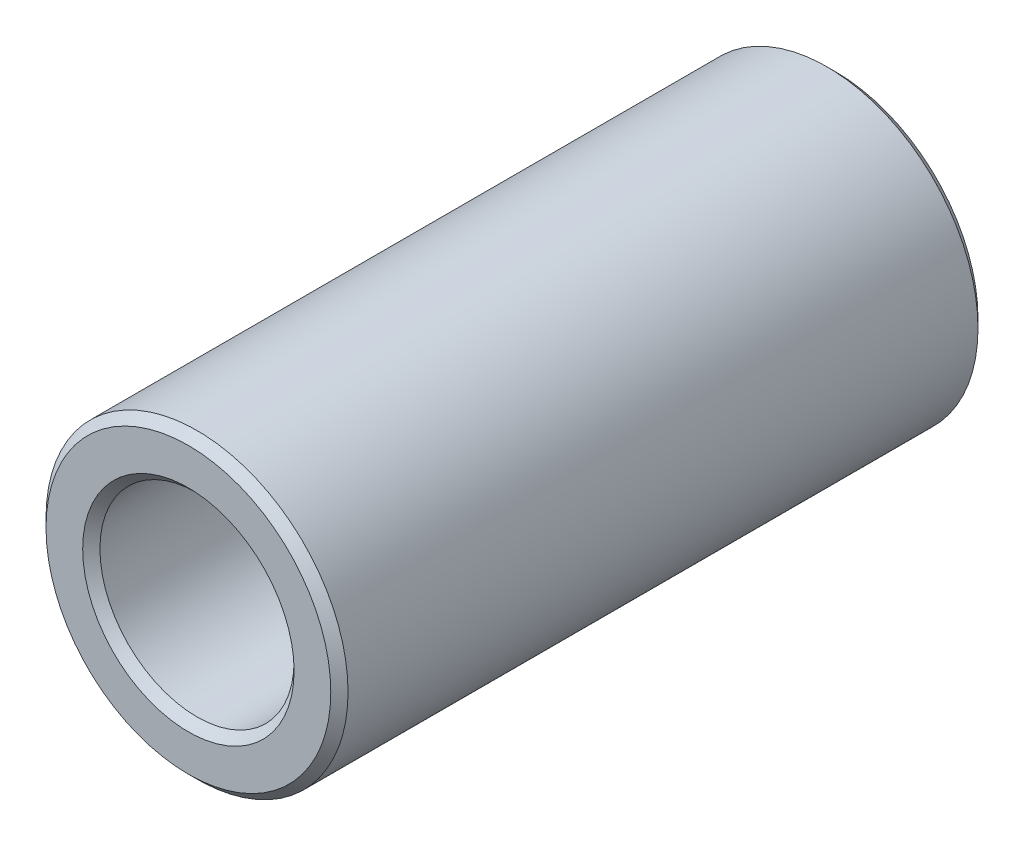
from build123d import *

# Parameters (mm, degrees)
SKETCH1_R           = 3.5
SKETCH1_R_2         = 2.25
BOSS_EXTRUDE1_DEPTH = 7.5
CHAMFER1_SIZE       = 0.2


with BuildPart() as part:
    # Sketch1 → Boss-Extrude1 (new, symmetric)
    with BuildSketch(Plane.XY):
        Circle(SKETCH1_R)
        Circle(SKETCH1_R_2, mode=Mode.SUBTRACT)
    extrude(amount=BOSS_EXTRUDE1_DEPTH, both=True)

    # Chamfer1
    chamfer1_edges = [part.edges().sort_by_distance(p)[0] for p in [
        (-3.5, 0, -7.5),
        (-3.5, 0, 7.5),
        (-2.25, 0, -7.5),
        (-2.25, 0, 7.5),
    ]]
    chamfer(chamfer1_edges, length=CHAMFER1_SIZE)


solid = part.part
